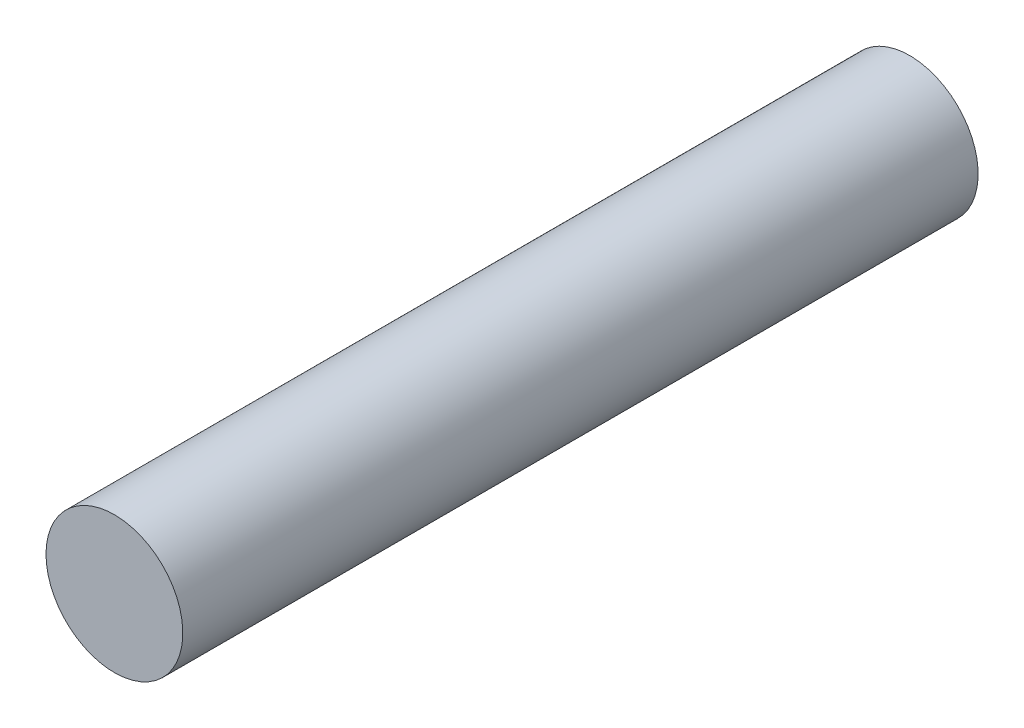
SolidWorks part; units mm, degrees
material "65Mn"
ref_plane "Front Plane" through (0, 0, 0) normal (0, 0, 1) x (1, 0, 0)
ref_plane "Top Plane" through (0, 0, 0) normal (0, 1, 0) x (1, 0, 0)
ref_plane "Right Plane" through (0, 0, 0) normal (1, 0, 0) x (0, 0, -1)
sketch "Sketch1" plane through (0, 0, 0) normal (0, 0, 1) x (1, 0, 0)
  circle A0 centre (0, 0) radius 4
  dimension "D1" = 8
extrude "Boss-Extrude1" add sketch "Sketch1" along normal blind 46.5
